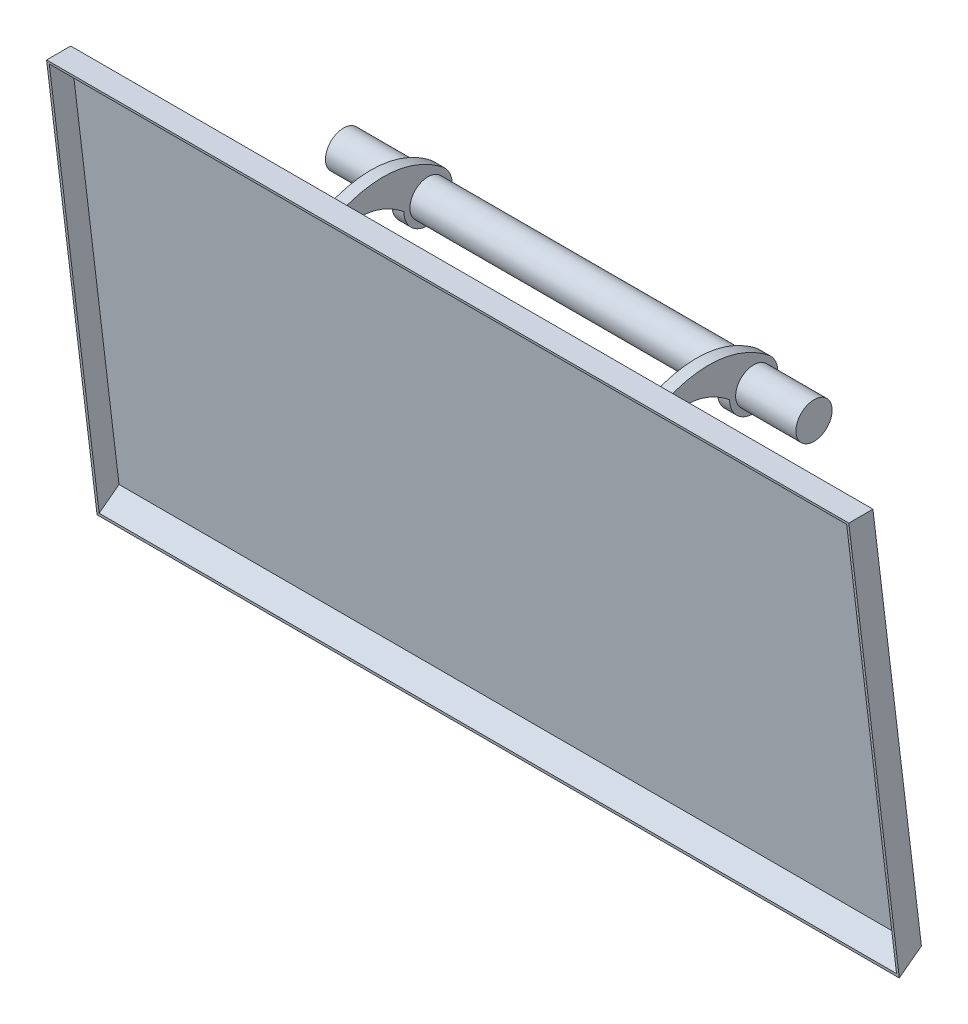
from build123d import *

# Parameters (mm, degrees)
BOSS_EXTRUDE1_DEPTH = 2
BOSS_EXTRUDE2_DEPTH = 661
BOSS_EXTRUDE3_DEPTH = 2
SKETCH4_R           = 15
BOSS_EXTRUDE4_DEPTH = 10
LPATTERN1_COUNT     = 2
LPATTERN1_PITCH     = 270
SKETCH5_R           = 15
BOSS_EXTRUDE5_DEPTH = 340
SKETCH6_R           = 15
BOSS_EXTRUDE6_DEPTH = 50


with BuildPart() as part:
    # Sketch1 → Boss-Extrude1 (new body)
    with BuildSketch(Plane(origin=(0, 0, 0), x_dir=(0, 0, -1), z_dir=(1, 0, 0))):
        Polygon((0, 0), (-20, 0), (21.83385642, -347.490904136), (40.177865273, -333.735493803), align=None)
    extrude(amount=BOSS_EXTRUDE1_DEPTH)

    # Sketch2 → Boss-Extrude2 (add)
    with BuildSketch(Plane.ZY):
        Polygon((0, 0), (20, 0), (19.759223301, -2), (1.773664518, -2), (-38.054187031, -332.828121742), (-21.557824554, -345.198058798), (-21.83385642, -347.490904136), (-40.177865273, -333.735493803), align=None)
    extrude(amount=BOSS_EXTRUDE2_DEPTH)

    # Sketch3 → Boss-Extrude3 (add)
    with BuildSketch(Plane.ZY.offset(661)):
        Polygon((20, 0), (0, 0), (-40.177865273, -333.735493803), (-21.83385642, -347.490904136), align=None)
    extrude(amount=BOSS_EXTRUDE3_DEPTH)

    # Sketch4 → Boss-Extrude4 (add)
    with BuildSketch(Plane(origin=(-195.5, 0, 0), x_dir=(0, 0, -1), z_dir=(1, 0, 0))):
        with BuildLine():
            Line((3.607407095, -29.964752484), (7.274393684, -60.424399152))
            Line((7.274393684, -60.424399152), (8.267224839, -60.304873847))
            ThreePointArc((8.267224839, -60.304873847), (12.936431276, -57.677699188), (14.380365793, -52.518378636))
            Line((14.380365793, -52.518378636), (12.826139197, -39.608270621))
            add(Edge.make_bspline(
                [(12.826139197, -39.608270621), (40.794384715, -27.323032004), (68.669426918, -49.466360803)],
                knots=[0, 0, 0, 1, 1, 1], degree=2))
            ThreePointArc((68.669426918, -49.466360803), (97.431993806, -67.44460937), (100.991169072, -33.712800243))
            add(Edge.make_bspline(
                [(3.607407095, -29.964752484), (33.423426205, -12.412570219), (69.250962672, -8.887006882), (100.991169072, -33.712800243)],
                knots=[0, 0, 0, 0, 1, 1, 1, 1], degree=3))
        make_face()
        with Locations((88.669426918, -49.466360803)):
            Circle(SKETCH4_R, mode=Mode.SUBTRACT)
    boss_extrude4 = extrude(amount=BOSS_EXTRUDE4_DEPTH)

    # LPattern1: Boss-Extrude4 ×2
    with Locations(*[(-i * LPATTERN1_PITCH, 0, 0) for i in range(1, LPATTERN1_COUNT)]):
        add(boss_extrude4)



with BuildPart() as body_2:
    # Sketch5 → Boss-Extrude5 (new body)
    with BuildSketch(Plane(origin=(-185.5, 0, 0), x_dir=(0, 0, -1), z_dir=(1, 0, 0))):
        with Locations((88.669426918, -49.466360803)):
            Circle(SKETCH5_R)
    extrude(amount=-BOSS_EXTRUDE5_DEPTH)


with BuildPart() as part_1:
    add(part.part)

    add(body_2.part)  # Boss-Extrude6 merges body 2
    # Sketch6 → Boss-Extrude6 (add)
    with BuildSketch(Plane(origin=(-185.5, 0, 0), x_dir=(0, 0, -1), z_dir=(1, 0, 0))):
        with Locations((88.669426918, -49.466360803)):
            Circle(SKETCH6_R)
    extrude(amount=BOSS_EXTRUDE6_DEPTH)


solid = part_1.part
